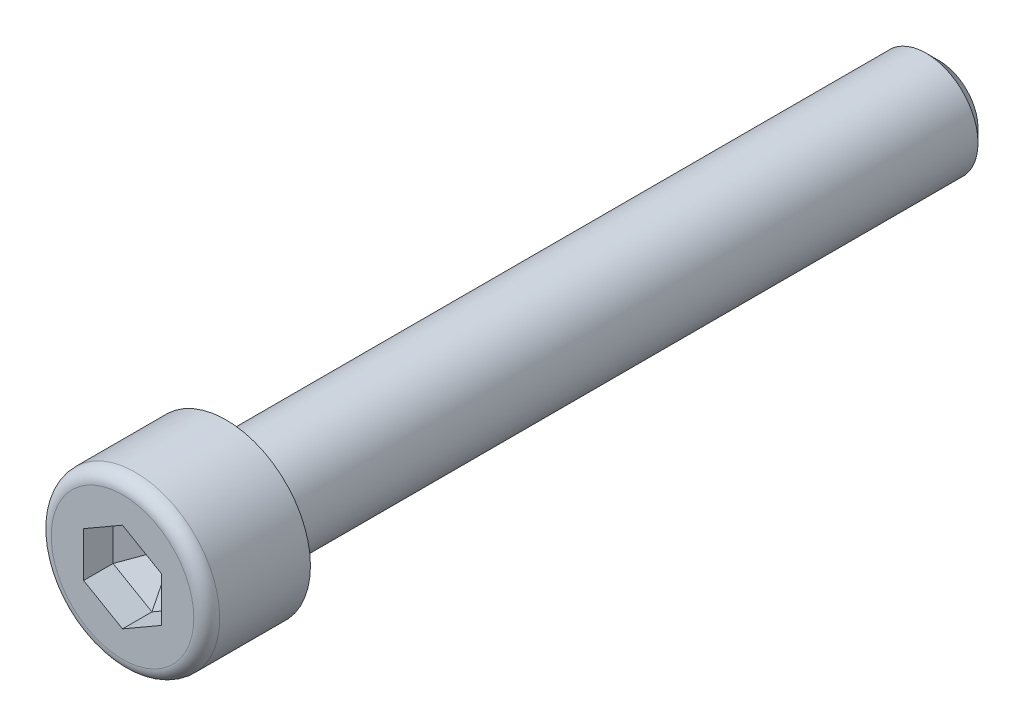
from build123d import *
from OCP.BRepFilletAPI import BRepFilletAPI_MakeChamfer

# Parameters (mm, degrees)
SKETCH1_R           = 6.5
BOSS_EXTRUDE1_DEPTH = 8
CUT_EXTRUDE1_DEPTH  = 4
SKETCH3_R           = 4
BOSS_EXTRUDE2_DEPTH = 55
CHAMFER1_SIZE       = 1
FILLET1_R           = 1
CHAMFER2_SIZE       = 1.729106628
CHAMFER2_SIZE2      = 2.994900532
FILLET2_R           = 0.1


with BuildPart() as part:
    # Sketch1 → Boss-Extrude1 (new body)
    with BuildSketch(Plane.XY):
        Circle(SKETCH1_R)
    extrude(amount=BOSS_EXTRUDE1_DEPTH)

    # Sketch2 → Cut-Extrude1 (cut)
    with BuildSketch(Plane.XY.offset(8)):
        Polygon((3, 1.732050808), (0, 3.464101615), (-3, 1.732050808), (-3, -1.732050808), (0, -3.464101615), (3, -1.732050808), align=None)
    extrude(amount=-CUT_EXTRUDE1_DEPTH, mode=Mode.SUBTRACT)

    # Sketch3 → Boss-Extrude2 (add)
    with BuildSketch(Plane(origin=(0, 0, 0), x_dir=(-1, 0, 0), z_dir=(0, 0, -1))):
        with Locations(Location((0, 0, 0), (0, 0, 180))):
            Circle(SKETCH3_R)
    extrude(amount=BOSS_EXTRUDE2_DEPTH)

    # Chamfer1
    chamfer1_edges = [part.edges().sort_by_distance(p)[0] for p in [
        (-4, 0, -55),
    ]]
    chamfer(chamfer1_edges, length=CHAMFER1_SIZE)

    # Fillet1
    fillet1_edges = [part.edges().sort_by_distance(p)[0] for p in [
        (-6.5, 0, 8),
    ]]
    fillet(fillet1_edges, radius=FILLET1_R)

    # Chamfer2: one chamfer whose edges measure the first distance from different faces: ONE call of the kernel's chamfer builder (chamfer() names one face for all edges)
    chamfer2_edges_1 = [part.edges().sort_by_distance(p)[0] for p in [
        (-1.5, 2.598076211, 4),
    ]]
    chamfer2_side_1 = [part.faces().sort_by_distance(p)[0] for p in [
        (-1.5, 2.598076211, 6),
    ]]
    chamfer2_edges_2 = [part.edges().sort_by_distance(p)[0] for p in [
        (1.5, 2.598076211, 4),
    ]]
    chamfer2_side_2 = [part.faces().sort_by_distance(p)[0] for p in [
        (1.5, 2.598076211, 6),
    ]]
    chamfer2_edges_3 = [part.edges().sort_by_distance(p)[0] for p in [
        (3, 0, 4),
    ]]
    chamfer2_side_3 = [part.faces().sort_by_distance(p)[0] for p in [
        (3, 0, 6),
    ]]
    chamfer2_edges_4 = [part.edges().sort_by_distance(p)[0] for p in [
        (1.5, -2.598076211, 4),
    ]]
    chamfer2_side_4 = [part.faces().sort_by_distance(p)[0] for p in [
        (1.5, -2.598076211, 6),
    ]]
    chamfer2_edges_5 = [part.edges().sort_by_distance(p)[0] for p in [
        (-1.5, -2.598076211, 4),
    ]]
    chamfer2_side_5 = [part.faces().sort_by_distance(p)[0] for p in [
        (-1.5, -2.598076211, 6),
    ]]
    chamfer2_edges_6 = [part.edges().sort_by_distance(p)[0] for p in [
        (-3, 0, 4),
    ]]
    chamfer2_side_6 = [part.faces().sort_by_distance(p)[0] for p in [
        (-3, 0, 6),
    ]]
    chamfer2 = BRepFilletAPI_MakeChamfer(part.part.solid().wrapped)
    for e in chamfer2_edges_1:
        chamfer2.Add(CHAMFER2_SIZE, CHAMFER2_SIZE2, e.wrapped, chamfer2_side_1[0].wrapped)  # the first distance lies on this face
    for e in chamfer2_edges_2:
        chamfer2.Add(CHAMFER2_SIZE, CHAMFER2_SIZE2, e.wrapped, chamfer2_side_2[0].wrapped)  # the first distance lies on this face
    for e in chamfer2_edges_3:
        chamfer2.Add(CHAMFER2_SIZE, CHAMFER2_SIZE2, e.wrapped, chamfer2_side_3[0].wrapped)  # the first distance lies on this face
    for e in chamfer2_edges_4:
        chamfer2.Add(CHAMFER2_SIZE, CHAMFER2_SIZE2, e.wrapped, chamfer2_side_4[0].wrapped)  # the first distance lies on this face
    for e in chamfer2_edges_5:
        chamfer2.Add(CHAMFER2_SIZE, CHAMFER2_SIZE2, e.wrapped, chamfer2_side_5[0].wrapped)  # the first distance lies on this face
    for e in chamfer2_edges_6:
        chamfer2.Add(CHAMFER2_SIZE, CHAMFER2_SIZE2, e.wrapped, chamfer2_side_6[0].wrapped)  # the first distance lies on this face
    add(Compound.cast(chamfer2.Shape()), mode=Mode.REPLACE)

    # Fillet2
    fillet2_edges = [part.edges().sort_by_distance(p)[0] for p in [
        (-4, 0, 0),
    ]]
    fillet(fillet2_edges, radius=FILLET2_R)


solid = part.part
